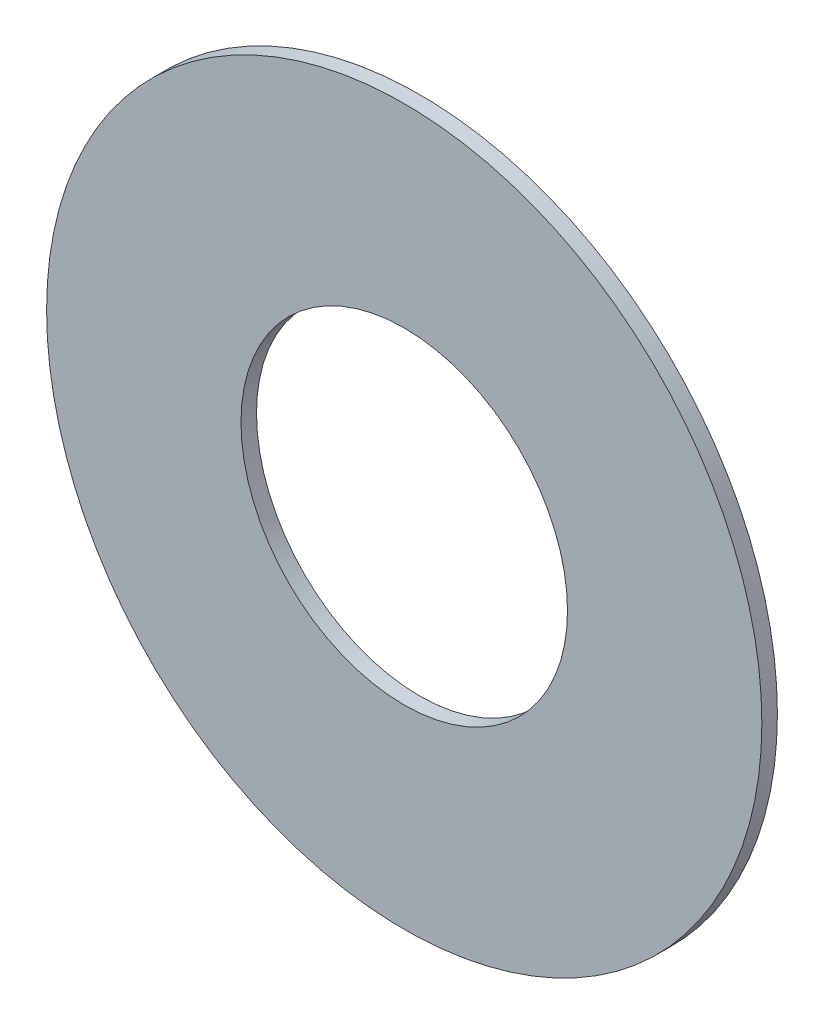
SolidWorks part; units mm, degrees
ref_plane "前视基准面" through (0, 0, 0) normal (0, 0, 1) x (1, 0, 0)
ref_plane "上视基准面" through (0, 0, 0) normal (0, 1, 0) x (1, 0, 0)
ref_plane "右视基准面" through (0, 0, 0) normal (1, 0, 0) x (0, 0, -1)
sketch "草图1" plane through (0, 0, 0) normal (0, 0, 1) x (1, 0, 0)
  circle A0 centre (0, 0) radius 23
  circle A1 centre (0, 0) radius 10.5
  dimension "D1" = 46
  dimension "D2" = 21
extrude "凸台-拉伸1" add sketch "草图1" along normal blind 1
